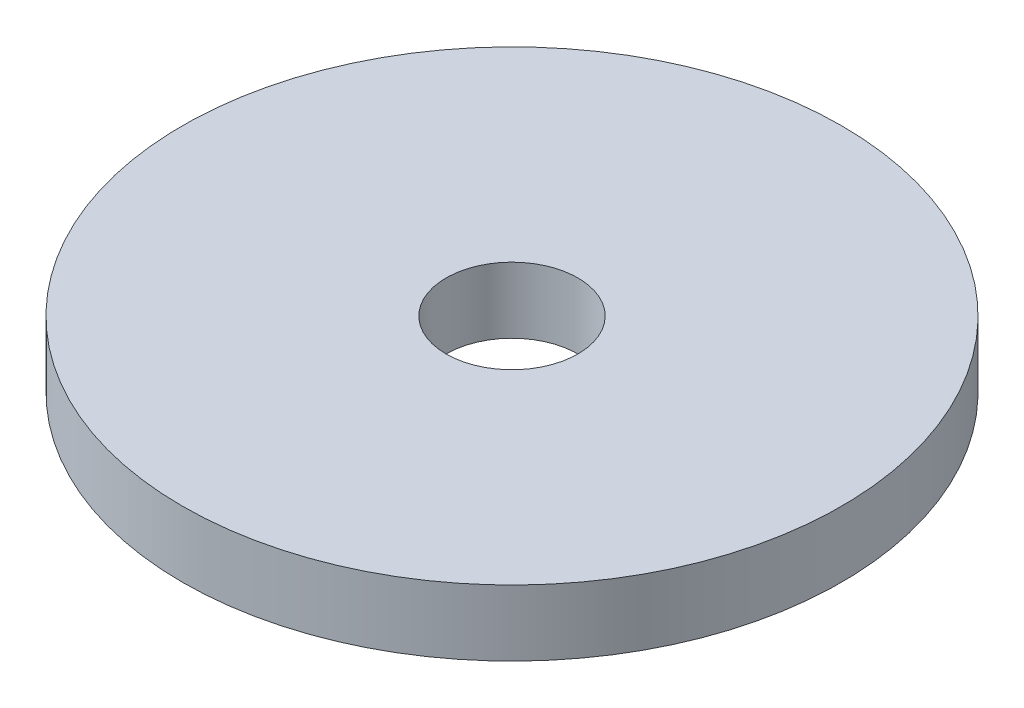
SolidWorks part; units mm, degrees
ref_plane "Front Plane" through (0, 0, 0) normal (0, 0, 1) x (1, 0, 0)
ref_plane "Top Plane" through (0, 0, 0) normal (0, 1, 0) x (1, 0, 0)
ref_plane "Right Plane" through (0, 0, 0) normal (1, 0, 0) x (0, 0, -1)
sketch "Sketch1" plane through (0, 0, 0) normal (0, 1, 0) x (1, 0, 0)
  circle A0 centre (0, 0) radius 10
  circle A1 centre (0, 0) radius 2
extrude "Boss-Extrude1" add sketch "Sketch1" along normal blind 2
